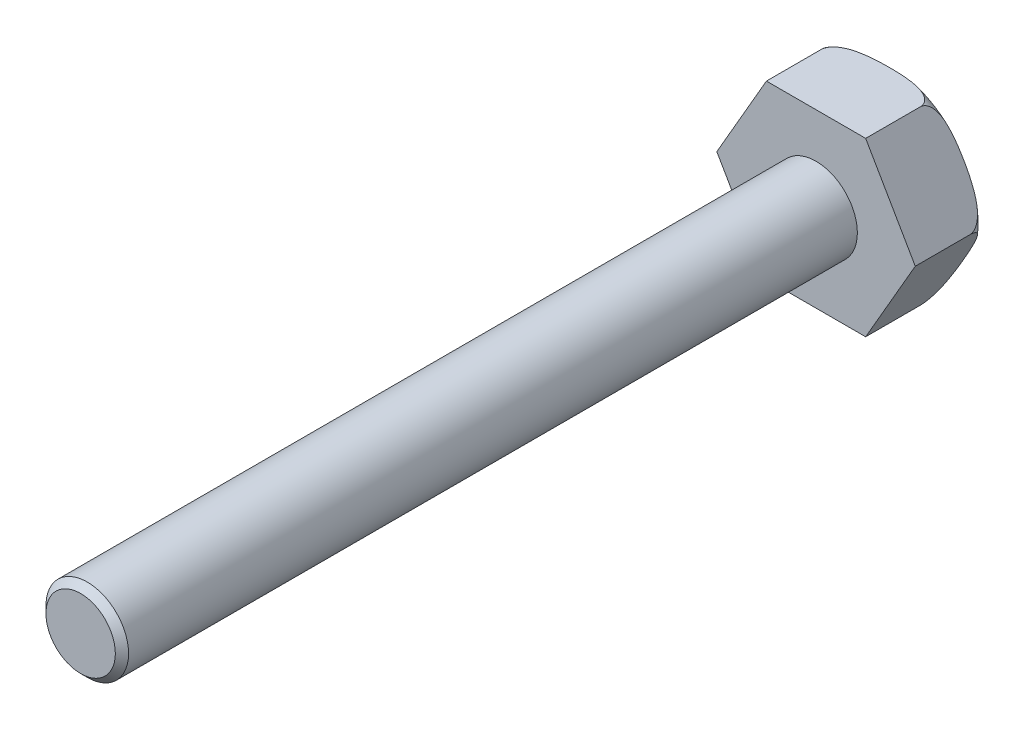
from build123d import *

# Parameters (mm, degrees)
BOSS_EXTRUDE1_DEPTH = 45
SKETCH4_R           = 25
BOSS_EXTRUDE2_DEPTH = 445
CHAMFER2_SIZE       = 4


with BuildPart() as part:
    # Sketch1 → Boss-Extrude1 (new body)
    with BuildSketch(Plane.XY):
        Polygon((30.022213998, -52), (60.044427996, 0), (30.022213998, 52), (-30.022213998, 52), (-60.044427996, 0), (-30.022213998, -52), align=None)
    extrude(amount=BOSS_EXTRUDE1_DEPTH)

    # Sketch3 → Cut-Revolve3 (revolve, cut)
    with BuildSketch(Plane(origin=(0, 0, 0), x_dir=(1, 0, 0), z_dir=(0, 1, 0))):
        with BuildLine():
            Line((-60.044427996, -12), (-60.044427996, 0))
            Line((-60.044427996, 0), (-48.044427996, 0))
            ThreePointArc((-48.044427996, 0), (-56.52970937, -3.514718626), (-60.044427996, -12))
        make_face()
    revolve(axis=Axis((0, 0, -19.888042613), (0, 0, 1)), mode=Mode.SUBTRACT)

    # Sketch4 → Boss-Extrude2 (add)
    with BuildSketch(Plane.XY.offset(45)):
        Circle(SKETCH4_R)
    extrude(amount=BOSS_EXTRUDE2_DEPTH)

    # Chamfer2
    chamfer2_edges = [part.edges().sort_by_distance(p)[0] for p in [
        (-25, 0, 490),
    ]]
    chamfer(chamfer2_edges, length=CHAMFER2_SIZE)


solid = part.part
